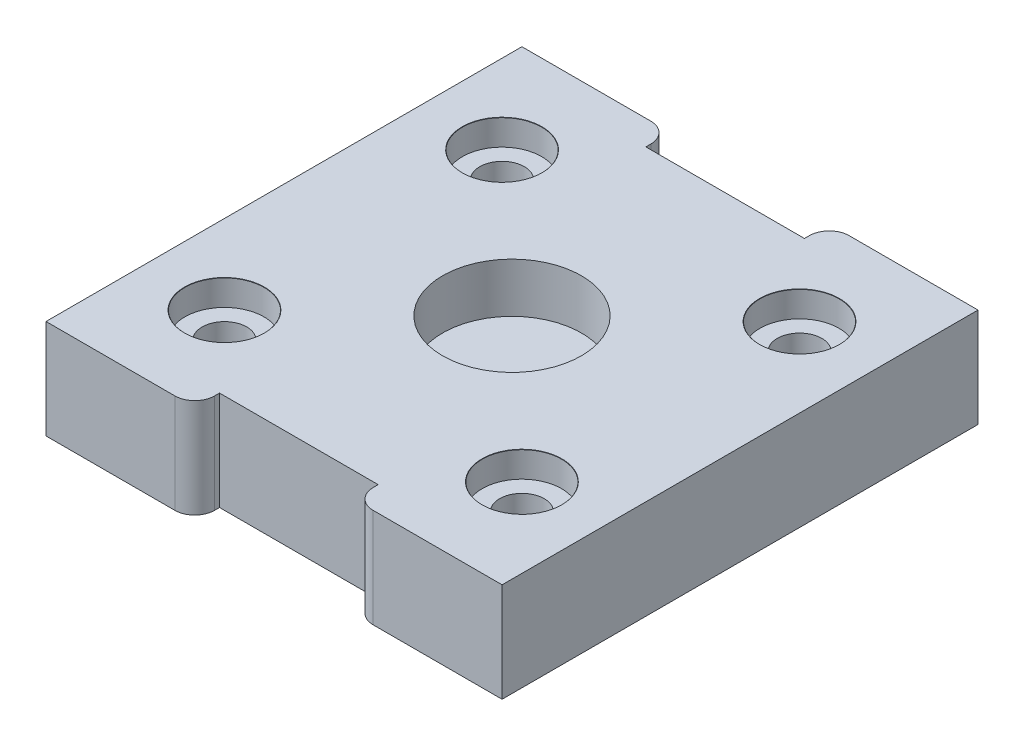
from build123d import *

# Parameters (mm, degrees)
SKETCH1_W                                  = 46
SKETCH1_H                                  = 10
BOSS_EXTRUDE1_DEPTH                        = 48
SKETCH2_W                                  = 16
SKETCH2_H                                  = 5
CUT_EXTRUDE1_DEPTH                         = 10
FILLET1_R                                  = 2
CBORE_FOR_M4_CHEESE_HEAD_SCREW1_AT_2_COUNT = 2
CBORE_FOR_M4_CHEESE_HEAD_SCREW1_AT_2_PITCH = 28
CBORE_FOR_M4_CHEESE_HEAD_SCREW1_AT_3_COUNT = 2
CBORE_FOR_M4_CHEESE_HEAD_SCREW1_AT_3_PITCH = 41.036569057
CBORE_FOR_M4_CHEESE_HEAD_SCREW1_AT_4_COUNT = 2
CBORE_FOR_M4_CHEESE_HEAD_SCREW1_AT_4_PITCH = 30
SKETCH6_R                                  = 7
CUT_EXTRUDE2_DEPTH                         = 5


with BuildPart() as part:
    # Sketch1 → Boss-Extrude1 (new body)
    with BuildSketch(Plane.XY):
        Rectangle(SKETCH1_W, SKETCH1_H)
    extrude(amount=BOSS_EXTRUDE1_DEPTH)

    # Sketch2 → Cut-Extrude1 (cut)
    with BuildSketch(Plane(origin=(0, 5, 0), x_dir=(1, 0, 0), z_dir=(0, 1, 0))):
        with Locations((0, -48)):
            Rectangle(SKETCH2_W, SKETCH2_H)
        Rectangle(SKETCH2_W, SKETCH2_H)
    extrude(amount=-CUT_EXTRUDE1_DEPTH, mode=Mode.SUBTRACT)

    # Fillet1
    fillet1_edges = [part.edges().sort_by_distance(p)[0] for p in [
        (-8, 0, 0),
        (8, 0, 0),
        (8, 0, 48),
        (-8, 0, 48),
    ]]
    fillet(fillet1_edges, radius=FILLET1_R)

    # Sketch4 → CBORE for M4 Cheese Head Screw1 (revolve, cut)
    with BuildSketch(Plane(origin=(-15, 5, 10), x_dir=(0, 0, 1), z_dir=(1, 0, 0))):
        Polygon((0, 0), (0, 11.351936393), (2.25, 10), (2.25, 2.6), (4, 2.6), (4, 0.025), (4.025, 0), align=None)
    cbore_for_m4_cheese_head_screw1 = revolve(axis=Axis((-15, 11.35, 10), (0, -1, 0)), mode=Mode.SUBTRACT)

    # CBORE for M4 Cheese Head Screw1 at 2: CBORE for M4 Cheese Head Screw1 ×2
    with Locations(*[(0, 0, i * CBORE_FOR_M4_CHEESE_HEAD_SCREW1_AT_2_PITCH) for i in range(1, CBORE_FOR_M4_CHEESE_HEAD_SCREW1_AT_2_COUNT)]):
        add(cbore_for_m4_cheese_head_screw1, mode=Mode.SUBTRACT)

    # CBORE for M4 Cheese Head Screw1 at 3: CBORE for M4 Cheese Head Screw1 ×2
    with Locations(*[Vector(0.731055268242869, 0, 0.6823182503600111) * (i * CBORE_FOR_M4_CHEESE_HEAD_SCREW1_AT_3_PITCH) for i in range(1, CBORE_FOR_M4_CHEESE_HEAD_SCREW1_AT_3_COUNT)]):
        add(cbore_for_m4_cheese_head_screw1, mode=Mode.SUBTRACT)

    # CBORE for M4 Cheese Head Screw1 at 4: CBORE for M4 Cheese Head Screw1 ×2
    with Locations(*[(i * CBORE_FOR_M4_CHEESE_HEAD_SCREW1_AT_4_PITCH, 0, 0) for i in range(1, CBORE_FOR_M4_CHEESE_HEAD_SCREW1_AT_4_COUNT)]):
        add(cbore_for_m4_cheese_head_screw1, mode=Mode.SUBTRACT)

    # Sketch6 → Cut-Extrude2 (cut)
    with BuildSketch(Plane(origin=(0, 5, 0), x_dir=(1, 0, 0), z_dir=(0, 1, 0))):
        with Locations(Location((0, -24, 0), (0, 0, 270))):
            Circle(SKETCH6_R)
    extrude(amount=-CUT_EXTRUDE2_DEPTH, mode=Mode.SUBTRACT)


solid = part.part
